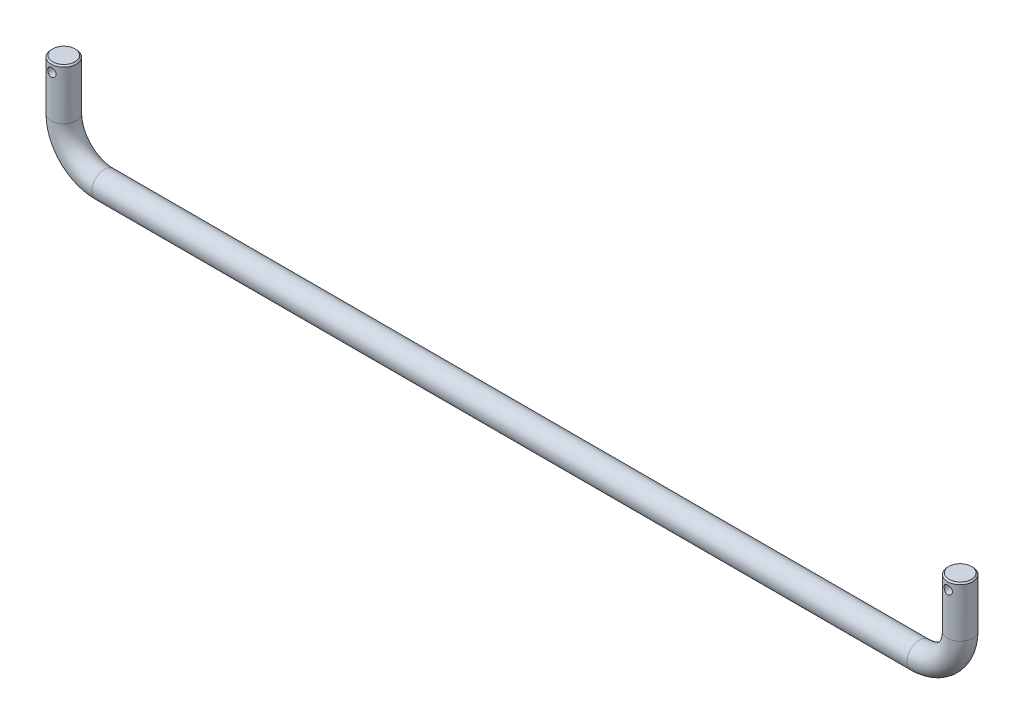
from build123d import *

# Parameters (mm, degrees)
SKETCH2_R               = 4.5
CUT_EXTRUDE1_DEPTH      = 10
CUT_EXTRUDE1_DEPTH_BACK = 10
SKETCH3_R               = 1.5
CHAMFER1_SIZE           = 0.5


with BuildPart() as part:
    # Sweep1: sweep along a path in Sketch1
    with BuildLine(Plane.XY) as sweep1_path:
        Line((0, 0), (0, -18))
        ThreePointArc((0, -18), (4.246951673, -28.253048327), (14.5, -32.5))
        Line((14.5, -32.5), (305.5, -32.5))
        ThreePointArc((305.5, -32.5), (315.753048327, -28.253048327), (320, -18))
        Line((320, -18), (320, 0))
    # Sketch2 → Sweep1 (sweep)
    with BuildSketch(Plane(origin=(0, 0, 0), x_dir=(1, 0, 0), z_dir=(0, 1, 0))):
        Circle(SKETCH2_R)
    sweep(path=sweep1_path.line)

    # Sketch3 → Cut-Extrude1 (cut, two sides: drawn at the far end of the back side and taken through both)
    with BuildSketch(Plane.XY.offset(-CUT_EXTRUDE1_DEPTH_BACK)):
        with Locations(Location((320, -3, 0), (0, 0, 180))):
            Circle(SKETCH3_R)
        with Locations(Location((0, -3, 0), (0, 0, 180))):
            Circle(SKETCH3_R)
    extrude(amount=CUT_EXTRUDE1_DEPTH + CUT_EXTRUDE1_DEPTH_BACK, mode=Mode.SUBTRACT)

    # Chamfer1
    chamfer1_edges = [part.edges().sort_by_distance(p)[0] for p in [
        (-4.5, 0, 0),
        (324.5, 0, 0),
    ]]
    chamfer(chamfer1_edges, length=CHAMFER1_SIZE)


solid = part.part
